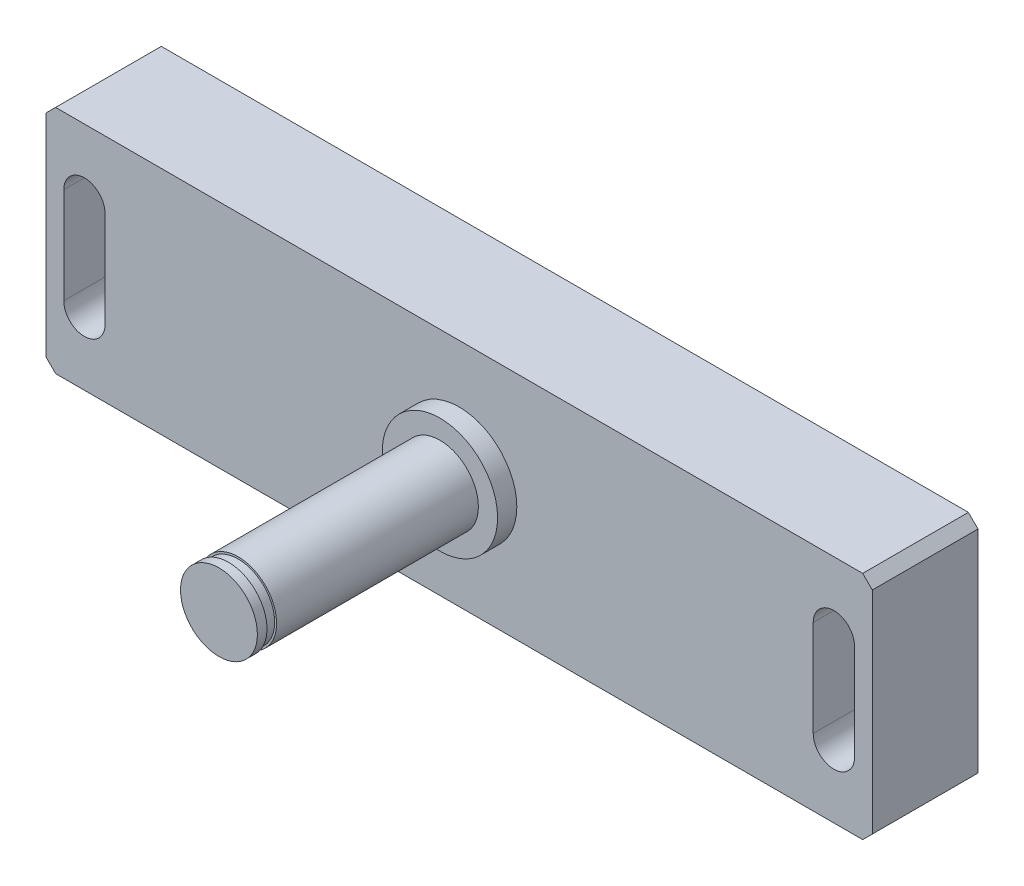
from build123d import *

# Parameters (mm, degrees)
SKETCH_1_W          = 86
SKETCH_1_H          = 24
EXTRUDE_1_DEPTH     = 5.5
SKETCH_2_R          = 4
EXTRUDE_2_DEPTH     = 3.5
SKETCH_3_R          = 4
EXTRUDE_3_DEPTH     = 21.5
CUT_EXTRUDE_4_DEPTH = 58.349803836
SKETCH_15_R         = 4
CUT_EXTRUDE_5_DEPTH = 9.999
SKETCH_4_W          = 0.2
SKETCH_4_H          = 1
SKETCH_16_R         = 2.9995
EXTRUDE_4_DEPTH     = 8.999
SKETCH_18_R         = 6
EXTRUDE_5_DEPTH     = 2
SKETCH_22_R         = 7.5
EXTRUDE_7_DEPTH     = 11
CHAMFER_1_SIZE      = 1


with BuildPart() as part:
    # 草图1 → 凸台-拉伸1 (new, symmetric)
    with BuildSketch(Plane.XY):
        Rectangle(SKETCH_1_W, SKETCH_1_H)
    extrude(amount=EXTRUDE_1_DEPTH, both=True)

    # 草图2 → 凸台-拉伸2 (add)
    with BuildSketch(Plane.XY.offset(5.5)):
        Circle(SKETCH_2_R)
    extrude(amount=EXTRUDE_2_DEPTH)

    # 草图3 → 凸台-拉伸3 (add)
    with BuildSketch(Plane.XY.offset(9)):
        Circle(SKETCH_3_R)
    extrude(amount=EXTRUDE_3_DEPTH)

    # 草图14 → 切除-拉伸4 (cut, through all)
    with BuildSketch(Plane(origin=(0, 0, -5.5), x_dir=(-1, 0, 0), z_dir=(0, 0, -1))):
        with BuildLine():
            Line((-36.85, 5), (-36.85, -5))
            ThreePointArc((-36.85, -5), (-39, -7.15), (-41.15, -5))
            Line((-41.15, -5), (-41.15, 5))
            ThreePointArc((-41.15, 5), (-39, 7.15), (-36.85, 5))
        make_face()
        with BuildLine():
            Line((36.85, 5), (36.85, -5))
            ThreePointArc((36.85, -5), (39, -7.15), (41.15, -5))
            Line((41.15, -5), (41.15, 5))
            ThreePointArc((41.15, 5), (39, 7.15), (36.85, 5))
        make_face()
    extrude(amount=-CUT_EXTRUDE_4_DEPTH, mode=Mode.SUBTRACT)

    # 草图15 → 切除-拉伸5 (cut)
    with BuildSketch(Plane(origin=(0, 0, -5.5), x_dir=(-1, 0, 0), z_dir=(0, 0, -1))):
        with Locations(Location((0, 0, 0), (0, 0, 180))):
            Circle(SKETCH_15_R)
    extrude(amount=-CUT_EXTRUDE_5_DEPTH, mode=Mode.SUBTRACT)

    # 草图4 → 切除-旋转1 (revolve, cut)
    with BuildSketch(Plane(origin=(0, 0, 0), x_dir=(1, 0, 0), z_dir=(0, 1, 0))):
        with Locations((-3.9, -29)):
            Rectangle(SKETCH_4_W, SKETCH_4_H)
    revolve(axis=Axis((0, 0, 0), (0, 0, 1)), mode=Mode.SUBTRACT)

    # 草图16 → 凸台-拉伸4 (add)
    with BuildSketch(Plane(origin=(0, 0, 4.499), x_dir=(-1, 0, 0), z_dir=(0, 0, -1))):
        Circle(SKETCH_16_R)
    extrude(amount=EXTRUDE_4_DEPTH)

    # 草图18 → 凸台-拉伸5 (add)
    with BuildSketch(Plane.XY.offset(5.5)):
        Circle(SKETCH_18_R)
    extrude(amount=EXTRUDE_5_DEPTH)

    # 草图22 → 凸台-拉伸7 (add)
    with BuildSketch(Plane(origin=(0, 0, -5.5), x_dir=(-1, 0, 0), z_dir=(0, 0, -1))):
        Circle(SKETCH_22_R)
    extrude(amount=-EXTRUDE_7_DEPTH)

    # 倒角1
    chamfer_1_edges = [part.edges().sort_by_distance(p)[0] for p in [
        (43, -12, 0),
        (-43, -12, 0),
        (-43, 12, 0),
        (43, 12, 0),
    ]]
    chamfer(chamfer_1_edges, length=CHAMFER_1_SIZE)


solid = part.part
